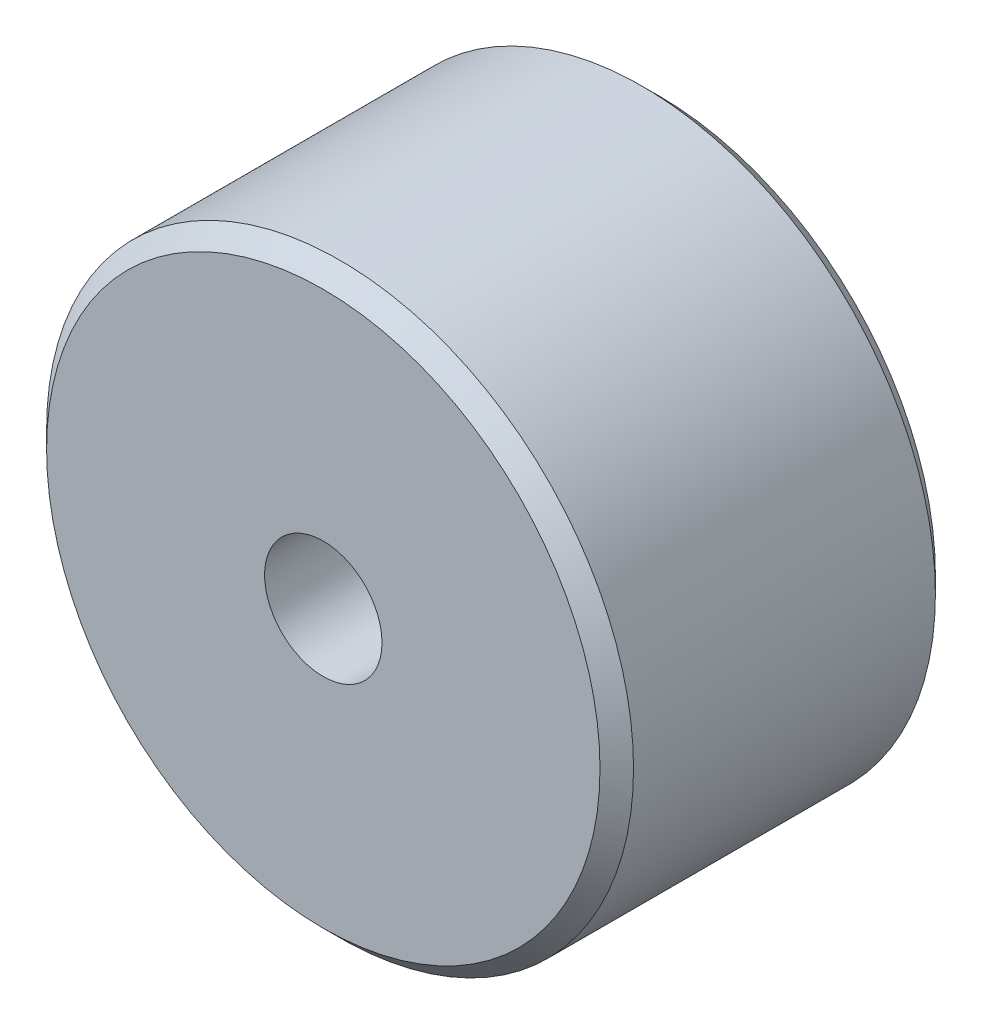
SolidWorks part; units mm, degrees
ref_plane "Front Plane" through (0, 0, 0) normal (0, 0, 1) x (1, 0, 0)
ref_plane "Top Plane" through (0, 0, 0) normal (0, 1, 0) x (1, 0, 0)
ref_plane "Right Plane" through (0, 0, 0) normal (1, 0, 0) x (0, 0, -1)
sketch "Sketch1" plane through (0, 0, 0) normal (0, 0, 1) x (1, 0, 0)
  circle A0 centre (0, 0) radius 35
  dimension "D1" = 70
extrude "Boss-Extrude1" add sketch "Sketch1" along normal blind 40
chamfer "Chamfer1" distance 2 angle 45 2 edges at (35, 0, 0) (35, 0, 40)
hole_wizard "M16 Tapped Hole1" positions "Sketch2" profile "Sketch4" tap size "M16" standard "GB" end condition through all
sketch "Sketch2" plane through (0, 0, 40) normal (0, 0, 1) x (1, 0, 0)
  point P0 (0, 0)
sketch "Sketch4" plane through (0, 0, 40) normal (1, 0, 0) x (0, -1, 0)
  line L0 (0, 0) -> (0, 40)
  line L1 (0, 40) -> (7, 40)
  line L2 (7, 40) -> (7, 0)
  line L5 (7, 0) -> (0, 0)
  line L11 (0, -6.35) -> (0, 107.95) construction
  dimension "通孔螺纹孔钻头直径" = 14
  dimension "通孔螺纹孔钻头深度" = 40
cosmetic thread "Cosmetic Thread1" parameters "D2"=16
